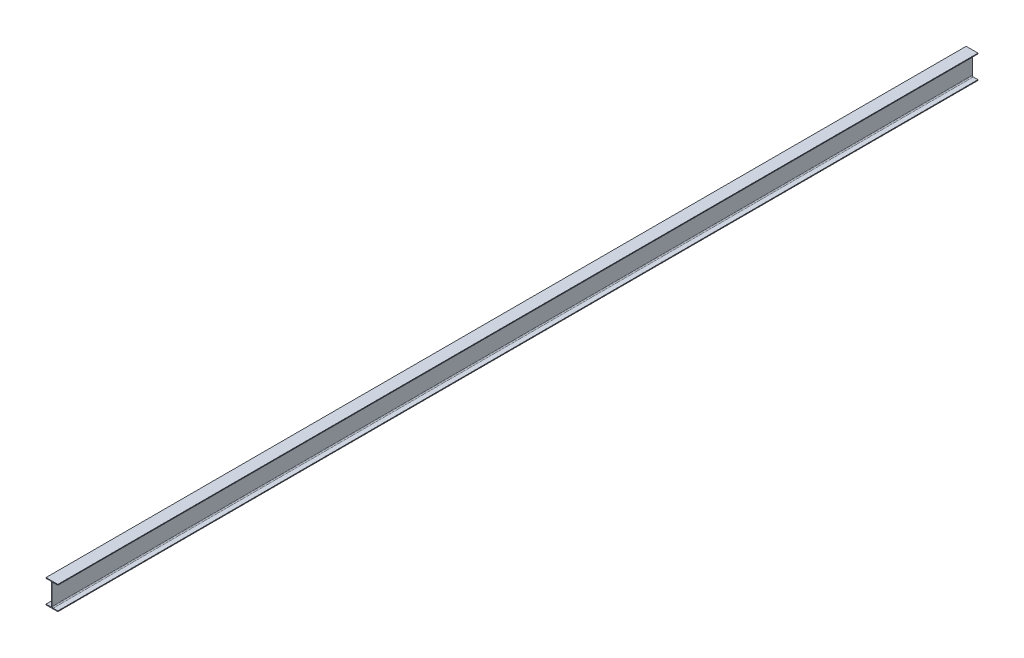
SolidWorks part; units mm, degrees
ref_plane "Front Plane" through (0, 0, 0) normal (0, 0, 1) x (1, 0, 0)
ref_plane "Top Plane" through (0, 0, 0) normal (0, 1, 0) x (1, 0, 0)
ref_plane "Right Plane" through (0, 0, 0) normal (1, 0, 0) x (0, 0, -1)
other "Configuration Table"
sketch "Sketch1" plane through (0, 0, 0) normal (0, 0, 1) x (1, 0, 0)
  line L0 (0, 0) -> (0, 300) construction
  line L1 (75, 0) -> (-75, 0)
  line L2 (-75, 0) -> (-75, 9)
  line L3 (-75, 9) -> (-16.25, 9)
  line L4 (3.25, 22) -> (3.25, 278)
  line L6 (-75, 291) -> (-75, 300)
  line L7 (-75, 300) -> (75, 300)
  line L8 (-3.25, 22) -> (-3.25, 278)
  line L9 (75, 291) -> (75, 300)
  line L10 (16.25, 291) -> (75, 291)
  line L11 (75, 9) -> (16.25, 9)
  line L12 (75, 0) -> (75, 9)
  line L13 (-16.25, 291) -> (-75, 291)
  arc A0 (16.25, 9) -> (3.25, 22) centre (16.25, 22) cw
  arc A1 (-3.25, 22) -> (-16.25, 9) centre (-16.25, 22) cw
  arc A2 (3.25, 278) -> (16.25, 291) centre (16.25, 278) cw
  arc A3 (-3.25, 278) -> (-16.25, 291) centre (-16.25, 278) ccw
  point P18 (3.25, 9)
  point P21 (-3.25, 9)
  point P24 (3.25, 291)
  point P27 (-3.25, 291)
  dimension "D6" = 13
  dimension "D1" = 300
  dimension "D2" = 150
  dimension "D3" = 6.5
  dimension "D4" = 9
  dimension "D5" = 9
extrude "Boss-Extrude1" add sketch "Sketch1" along normal blind 11647
